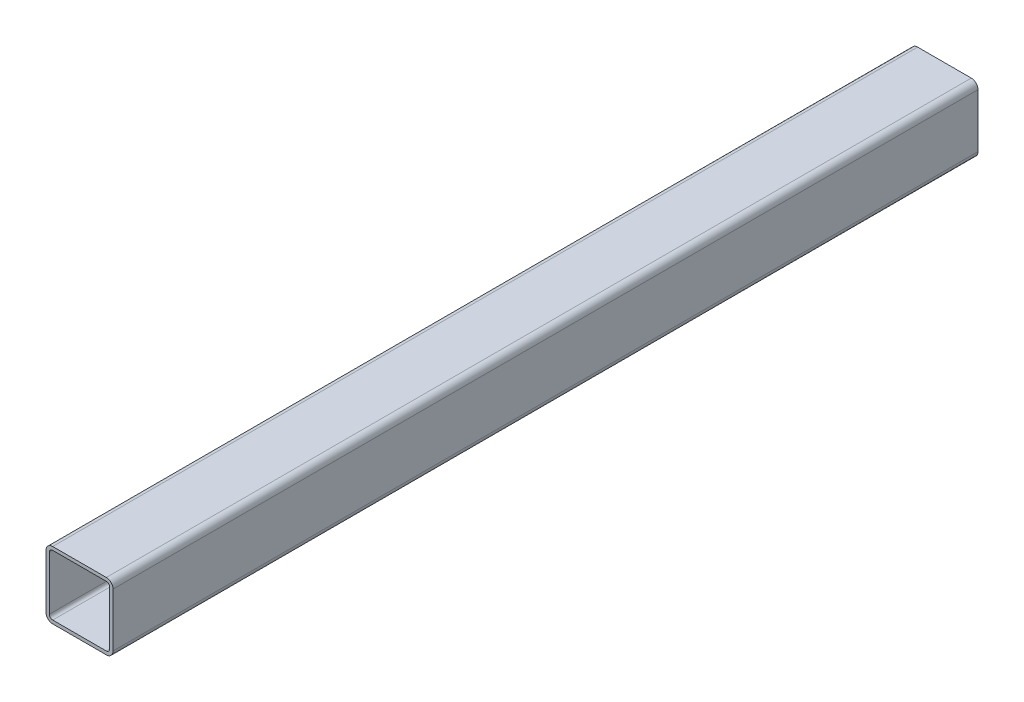
SolidWorks part; units mm, degrees
ref_plane "Front Plane" through (0, 0, 0) normal (0, 0, 1) x (1, 0, 0)
ref_plane "Top Plane" through (0, 0, 0) normal (0, 1, 0) x (1, 0, 0)
ref_plane "Right Plane" through (0, 0, 0) normal (1, 0, 0) x (0, 0, -1)
sketch "Sketch 1" plane through (0, 0, 0) normal (0, 0, 1) x (1, 0, 0)
  line L0 (0, 96.8978) -> (0, -107.4818) construction
  line L1 (-129.1971, 0) -> (137.9562, 0) construction
  line L2 (0, 50) -> (-40, 50)
  line L3 (-50, 40) -> (-50, 0)
  line L4 (0, 45) -> (-40, 45)
  line L5 (-45, 40) -> (-45, 0)
  line L6 (-45, -40) -> (-45, 0)
  line L7 (40, -45) -> (-40, -45)
  line L8 (-50, -40) -> (-50, 0)
  line L9 (40, -50) -> (-40, -50)
  line L10 (50, -40) -> (50, 0)
  line L11 (45, -40) -> (45, 0)
  line L12 (45, 40) -> (45, 0)
  line L13 (0, 45) -> (40, 45)
  line L14 (50, 40) -> (50, 0)
  line L15 (0, 50) -> (40, 50)
  arc A0 (-40, 50) -> (-50, 40) centre (-40, 40) ccw
  arc A1 (-40, 45) -> (-45, 40) centre (-40, 40) ccw
  arc A2 (-40, -45) -> (-45, -40) centre (-40, -40) cw
  arc A3 (-40, -50) -> (-50, -40) centre (-40, -40) cw
  arc A4 (40, -50) -> (50, -40) centre (40, -40) ccw
  arc A5 (40, -45) -> (45, -40) centre (40, -40) ccw
  arc A6 (40, 45) -> (45, 40) centre (40, 40) cw
  arc A7 (40, 50) -> (50, 40) centre (40, 40) cw
  point P34 (0, -50)
  point P35 (0, -45)
  dimension "D3" = 10
  dimension "D1" = 100
  dimension "D2" = 100
  dimension "D4" = 5
extrude "Boss-Extrude 1" add sketch "Sketch 1" along normal mid plane 1290
